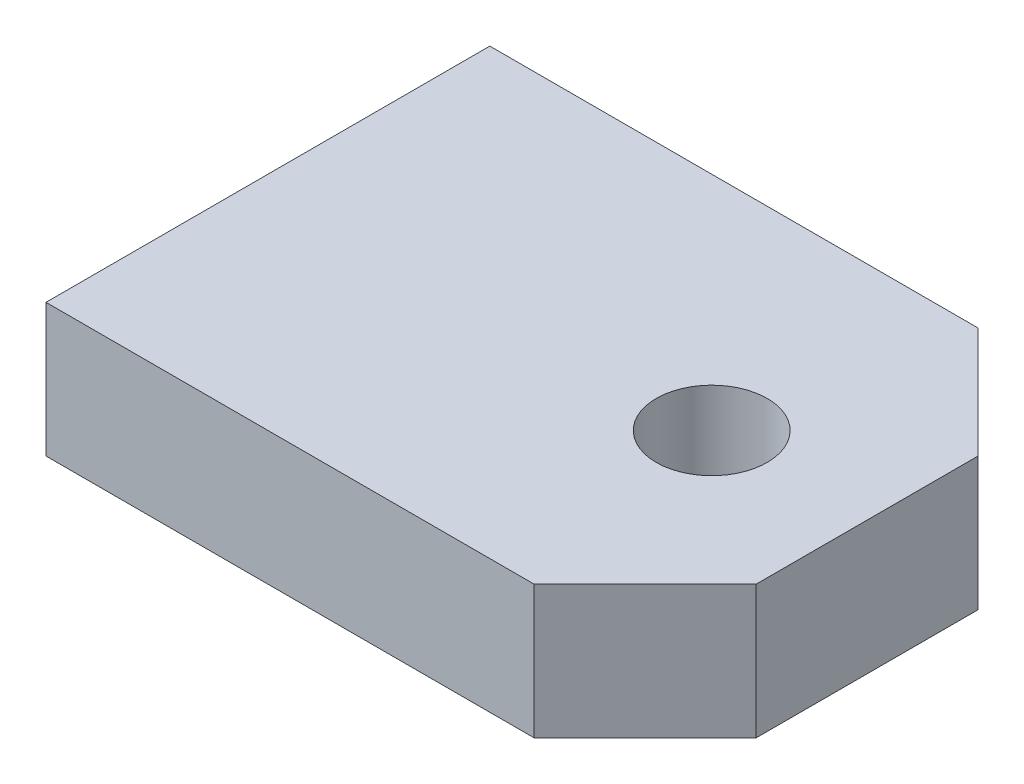
from build123d import *

# Parameters (mm, degrees)
SKETCH_1_W             = 27
SKETCH_1_H             = 6
EXTRUDE_1_DEPTH        = 20
HOLE_WIZARD_M6_1_D     = 5
HOLE_WIZARD_M6_1_DEPTH = 15
HOLE_WIZARD_M6_1_TIP   = 1.502151548
CHAMFER_1_SIZE         = 5


with BuildPart() as part:
    # 草图1 → 凸台-拉伸1 (new body)
    with BuildSketch(Plane.XY):
        Rectangle(SKETCH_1_W, SKETCH_1_H)
    extrude(amount=EXTRUDE_1_DEPTH)

    # M6 螺纹孔1
    with Locations(Plane(origin=(0, 3, 0), x_dir=(1, 0, 0), z_dir=(0, 1, 0))):
        with Locations((6.5, -10)):
            Hole(HOLE_WIZARD_M6_1_D / 2, depth=HOLE_WIZARD_M6_1_DEPTH)
            with Locations((0, 0, -(HOLE_WIZARD_M6_1_DEPTH + HOLE_WIZARD_M6_1_TIP / 2))):  # 118° drill point
                Cone(0, HOLE_WIZARD_M6_1_D / 2, HOLE_WIZARD_M6_1_TIP, mode=Mode.SUBTRACT)

    # 倒角1
    chamfer_1_edges = [part.edges().sort_by_distance(p)[0] for p in [
        (13.5, 0, 20),
        (13.5, 0, 0),
    ]]
    chamfer(chamfer_1_edges, length=CHAMFER_1_SIZE)


solid = part.part
